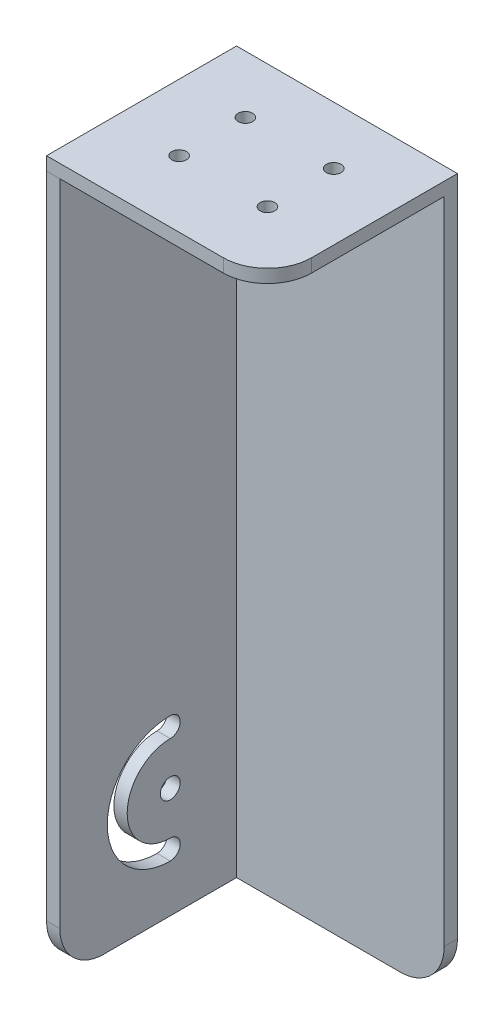
from build123d import *

# Parameters (mm, degrees)
SKETCH_1_W                  = 50
SKETCH_1_H                  = 160
EXTRUDE_1_DEPTH             = 3
SKETCH_2_W                  = 50
SKETCH_2_H                  = 3
EXTRUDE_2_DEPTH             = 40
SKETCH_5_W                  = 40
SKETCH_5_H                  = 157
EXTRUDE_3_DEPTH             = 3
SKETCH_6_R                  = 2.25
CUT_EXTRUDE_1_DEPTH         = 10
SKETCH_8_W                  = 1.65
SKETCH_8_H                  = 160
HOLE_WIZARD_M4_1_AT_2_COUNT = 2
HOLE_WIZARD_M4_1_AT_2_PITCH = 20
HOLE_WIZARD_M4_1_AT_3_COUNT = 2
HOLE_WIZARD_M4_1_AT_3_PITCH = 15
HOLE_WIZARD_M4_1_AT_4_COUNT = 2
HOLE_WIZARD_M4_1_AT_4_PITCH = 25
FILLET_1_R                  = 10
FILLET_2_R                  = 10


with BuildPart() as part:
    # 草图1 → 凸台-拉伸1 (new body)
    with BuildSketch(Plane.XY):
        Rectangle(SKETCH_1_W, SKETCH_1_H)
    extrude(amount=EXTRUDE_1_DEPTH)

    # 草图2 → 凸台-拉伸2 (add)
    with BuildSketch(Plane.XY.offset(3)):
        with Locations((0, 78.5)):
            Rectangle(SKETCH_2_W, SKETCH_2_H)
    extrude(amount=EXTRUDE_2_DEPTH)

    # 草图8 → M4 螺纹孔1 (revolve, cut)
    with BuildSketch(Plane(origin=(-10, 80, 13), x_dir=(0, 0, 1), z_dir=(1, 0, 0))):
        with Locations((0.825, 80)):
            Rectangle(SKETCH_8_W, SKETCH_8_H)
    hole_wizard_m4_1 = revolve(axis=Axis((-10, 86.35, 13), (0, -1, 0)), mode=Mode.SUBTRACT)

    # M4 螺纹孔1 at 2: M4 螺纹孔1 ×2
    with Locations(*[(i * HOLE_WIZARD_M4_1_AT_2_PITCH, 0, 0) for i in range(1, HOLE_WIZARD_M4_1_AT_2_COUNT)]):
        add(hole_wizard_m4_1, mode=Mode.SUBTRACT)

    # M4 螺纹孔1 at 3: M4 螺纹孔1 ×2
    with Locations(*[(0, 0, i * HOLE_WIZARD_M4_1_AT_3_PITCH) for i in range(1, HOLE_WIZARD_M4_1_AT_3_COUNT)]):
        add(hole_wizard_m4_1, mode=Mode.SUBTRACT)

    # M4 螺纹孔1 at 4: M4 螺纹孔1 ×2
    with Locations(*[Vector(0.8000000000000002, 0, 0.5999999999999999) * (i * HOLE_WIZARD_M4_1_AT_4_PITCH) for i in range(1, HOLE_WIZARD_M4_1_AT_4_COUNT)]):
        add(hole_wizard_m4_1, mode=Mode.SUBTRACT)

    # 圆角1
    fillet_1_edges = [part.edges().sort_by_distance(p)[0] for p in [
        (25, 78.5, 43),
        (25, -80, 1.5),
    ]]
    fillet(fillet_1_edges, radius=FILLET_1_R)


with BuildPart() as body_2:
    # 草图5 → 凸台-拉伸3 (new body)
    with BuildSketch(Plane.ZY.offset(25)):
        with Locations((23, -1.5)):
            Rectangle(SKETCH_5_W, SKETCH_5_H)
    extrude(amount=-EXTRUDE_3_DEPTH)

    # 草图6 → 切除-拉伸1 (cut)
    with BuildSketch(Plane(origin=(-22, 0, 0), x_dir=(0, 0, -1), z_dir=(1, 0, 0))):
        with Locations(Location((-18, -55, 0), (0, 0, 90))):
            Circle(SKETCH_6_R)
        with BuildLine():
            ThreePointArc((-18, -40.75), (-32.25, -55), (-18, -69.25))
            ThreePointArc((-18, -69.25), (-15.75, -67), (-18, -64.75))
            ThreePointArc((-18, -64.75), (-27.75, -55), (-18, -45.25))
            ThreePointArc((-18, -45.25), (-15.75, -43), (-18, -40.75))
        make_face()
    extrude(amount=-CUT_EXTRUDE_1_DEPTH, mode=Mode.SUBTRACT)

    # 圆角2
    fillet_2_edges = [body_2.edges().sort_by_distance(p)[0] for p in [
        (-23.5, -80, 43),
    ]]
    fillet(fillet_2_edges, radius=FILLET_2_R)


solid = Compound([part.part, body_2.part])
